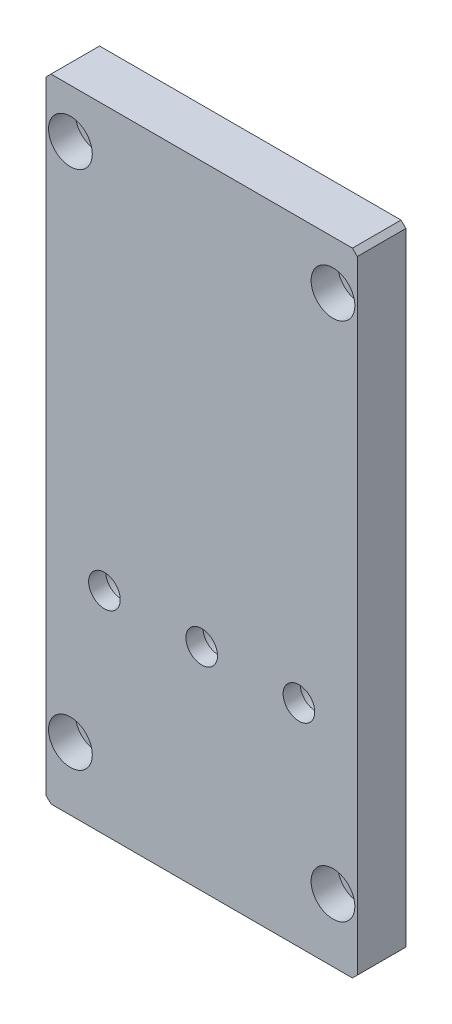
from build123d import *

# Parameters (mm, degrees)
SKETCH_1_W                  = 64
SKETCH_1_H                  = 130
EXTRUDE_1_DEPTH             = 10
HOLE_WIZARD_0_D             = 5.5
HOLE_WIZARD_0_CBORE_D       = 9
HOLE_WIZARD_0_CBORE_DEPTH   = 5.5
HOLE_WIZARD_C_1_D           = 6.5
HOLE_WIZARD_C_1_CBORE_D     = 12
HOLE_WIZARD_C_1_CBORE_DEPTH = 6.5
CHAMFER_1_SIZE              = 1


with BuildPart() as part:
    # 草图1 → 凸台-拉伸1 (new body)
    with BuildSketch(Plane.XY):
        with Locations((10, -65)):
            Rectangle(SKETCH_1_W, SKETCH_1_H)
    extrude(amount=EXTRUDE_1_DEPTH)

    # 打孔尺寸根据内六角圆柱头螺钉的类型0 (through all)
    with Locations(Plane.XY.offset(10)):
        with Locations((-17, -10), (37, -10), (-17, -117), (37, -117)):
            CounterBoreHole(HOLE_WIZARD_0_D / 2, HOLE_WIZARD_0_CBORE_D / 2, HOLE_WIZARD_0_CBORE_DEPTH)

    # 打孔尺寸根据六角头螺栓 C 级的类型1 (through all)
    with Locations(Plane(origin=(0, 0, 0), x_dir=(-1, 0, 0), z_dir=(0, 0, -1))):
        with Locations((10, -86.5), (-10, -86.5), (-30, -86.5)):
            CounterBoreHole(HOLE_WIZARD_C_1_D / 2, HOLE_WIZARD_C_1_CBORE_D / 2, HOLE_WIZARD_C_1_CBORE_DEPTH)

    # 倒角1
    chamfer_1_edges = [part.edges().sort_by_distance(p)[0] for p in [
        (-22, 0, 5),
        (42, 0, 5),
        (42, -130, 5),
        (-22, -130, 5),
    ]]
    chamfer(chamfer_1_edges, length=CHAMFER_1_SIZE)


solid = part.part
